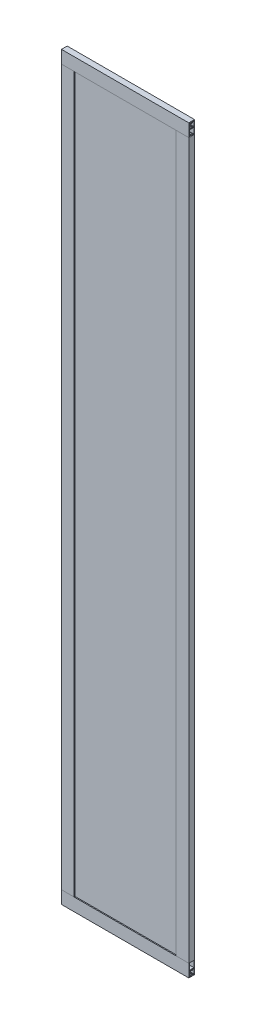
SolidWorks part; units mm, degrees
material "铝合金板 LF5"
ref_plane "前视基准面" through (0, 0, 0) normal (0, 0, 1) x (1, 0, 0)
ref_plane "上视基准面" through (0, 0, 0) normal (0, 1, 0) x (1, 0, 0)
ref_plane "右视基准面" through (0, 0, 0) normal (1, 0, 0) x (0, 0, -1)
sketch "草图1" plane through (0, 0, 0) normal (0, 0, 1) x (1, 0, 0)
  line L1 (-199.25, 1158.5) -> (199.25, 1158.5)
  line L2 (-199.25, 1158.5) -> (-199.25, -1158.5)
  line L3 (-199.25, -1158.5) -> (199.25, -1158.5)
  line L4 (199.25, 1158.5) -> (199.25, -1158.5)
  line L5 (-199.25, 1158.5) -> (199.25, -1158.5) construction
  line L6 (-199.25, -1158.5) -> (199.25, 1158.5) construction
  point P0 (0, 0)
other "自定义 玻璃外框(1)"
ref_plane "基准面4" through (-199.25, 1158.5, 0) normal (1, 0, 0) x (0, 0, -1)
sketch "Sketch1" plane through (-199.25, 1158.5, 0) normal (1, 0, 0) x (0, 0, -1)
  line L8 (-1.3416, -18) -> (1.3416, -18)
  line L9 (2.6401, -18) -> (7, -18)
  line L10 (7, -18) -> (7, -3)
  line L11 (7, -3) -> (2.6401, -3)
  line L12 (1.3416, -3) -> (-1.3416, -3)
  line L13 (-2.6401, -3) -> (-7, -3)
  line L14 (-7, -3) -> (-7, -18)
  line L15 (-7, -18) -> (-2.6401, -18)
  line L17 (7, -38.5) -> (5.9, -38.5)
  line L18 (5.9, -38.5) -> (5.9, -40)
  line L19 (5.9, -40) -> (7, -40)
  line L20 (7, -40) -> (9, -40)
  line L21 (9, -40) -> (9, 0)
  line L22 (9, 0) -> (-9, 0)
  line L23 (-9, 0) -> (-9, -40)
  line L24 (-9, -40) -> (-7, -40)
  line L25 (-7, -40) -> (-5.9, -40)
  line L26 (-5.9, -40) -> (-5.9, -38.5)
  line L27 (-5.9, -38.5) -> (-7, -38.5)
  line L28 (-7, -38.5) -> (-7, -20)
  line L29 (-7, -20) -> (7, -20)
  line L30 (7, -20) -> (7, -38.5)
  arc A0 (2.0506, -14.7494) -> (1.2728, -15.5272) centre (1.6617, -15.1383) ccw
  arc A1 (2.6401, -18) -> (2.0506, -14.7494) centre (0, -16.8) ccw
  arc A2 (2.0506, -6.2506) -> (2.6401, -3) centre (0, -4.2) ccw
  arc A3 (1.2728, -5.4728) -> (2.0506, -6.2506) centre (1.6617, -5.8617) ccw
  arc A4 (1.2728, -5.4728) -> (1.3416, -3) centre (0, -4.2) ccw
  arc A5 (-1.3416, -3) -> (-1.2728, -5.4728) centre (0, -4.2) ccw
  arc A6 (-2.0506, -6.2506) -> (-1.2728, -5.4728) centre (-1.6617, -5.8617) ccw
  arc A7 (-2.6401, -3) -> (-2.0506, -6.2506) centre (0, -4.2) ccw
  arc A8 (-2.0506, -14.7494) -> (-2.6401, -18) centre (0, -16.8) ccw
  arc A9 (-1.2728, -15.5272) -> (-2.0506, -14.7494) centre (-1.6617, -15.1383) ccw
  arc A10 (-1.2728, -15.5272) -> (-1.3416, -18) centre (0, -16.8) ccw
  arc A11 (1.3416, -18) -> (1.2728, -15.5272) centre (0, -16.8) ccw
  point P0 (0, 0)
sketch "草图2" plane through (0, 0, 9) normal (0, 0, 1) x (1, 0, 0)
  line L0 (-159.25, 1118.5) -> (159.25, -1118.5) construction
  line L1 (199.25, -1158.5) -> (-199.25, -1158.5) construction
  line L2 (-176.25, 1135.5) -> (176.25, 1135.5)
  line L3 (-176.25, 1135.5) -> (-176.25, -1135.5)
  line L4 (-176.25, -1135.5) -> (176.25, -1135.5)
  line L5 (176.25, 1135.5) -> (176.25, -1135.5)
  line L6 (-176.25, 1135.5) -> (176.25, -1135.5) construction
  line L7 (-176.25, -1135.5) -> (176.25, 1135.5) construction
  line L8 (199.25, -1118.5) -> (199.25, 1118.5) construction
  point P4 (0, 0)
  dimension "D1" = 23
  dimension "D2" = 23
  dimension "D3" = 352.5
  dimension "D4" = 2271
extrude "凸台-拉伸1" add sketch "草图2" against normal blind 10 from offset 3.1 separate body offset against normal yes
equation "\"A\" =1195"
equation "\"B\" =1155"
equation "\"CH\" = 2300"
equation "\"OP\" =750"
equation "\"OPH\" = 2100"
equation "\"QB\" = 50"
equation "\"DK\" = 40"
equation "\"WCOP\" =0"
equation "\"HCOP\" =4"
equation "\"FJ\" = 2"
equation "\"DH\" = 16"
equation "\"LG\" = 1"
equation "\"DD\" = 2"
equation "\"C\" =545"
equation "\"PX\" =-75"
equation "\"LZ\" = 350"
equation "\"LJ\" = 1158"
equation "\"LLK\" = 310"
equation "\"FS\" = 0"
equation "\"后玻璃框（纵）\"= \"CH\" + \"DH\" + 1"
equation "\"后玻璃框（横向）\"= 0'见轿厢"
equation "\"D2@草图1\"=\"后玻璃框（纵）\""
